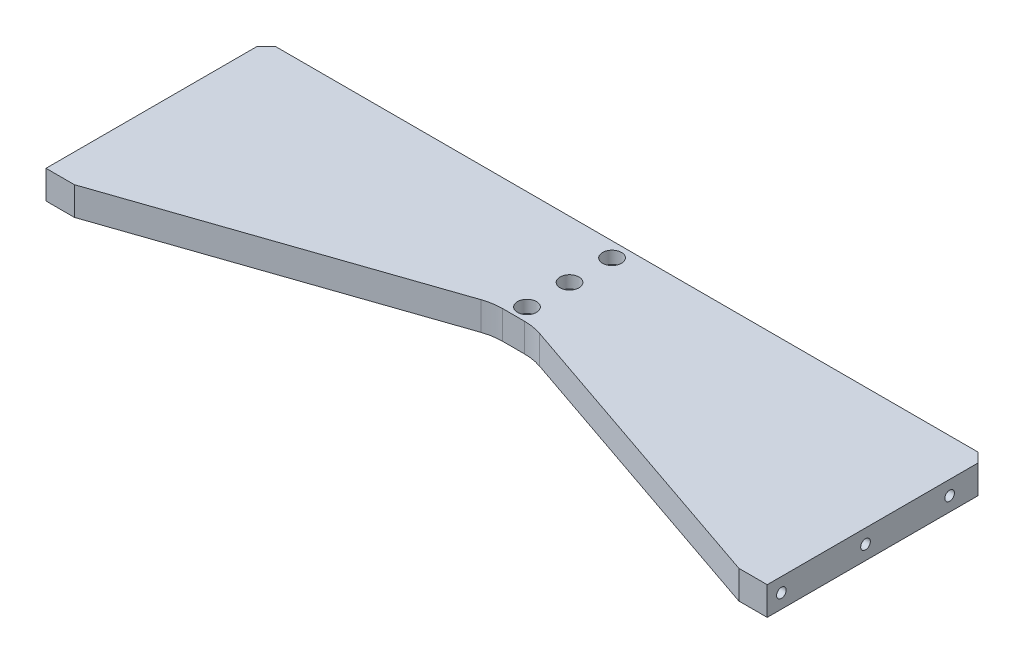
SolidWorks part; units mm, degrees
material "普通碳钢"
ref_plane "前视基准面" through (0, 0, 0) normal (0, 0, 1) x (1, 0, 0)
ref_plane "上视基准面" through (0, 0, 0) normal (0, 1, 0) x (1, 0, 0)
ref_plane "右视基准面" through (0, 0, 0) normal (1, 0, 0) x (0, 0, -1)
sketch "草图1" plane through (0, 0, 0) normal (0, 1, 0) x (1, 0, 0)
  line L1 (-381.5, -116.5) -> (381.5, -116.5)
  line L2 (-381.5, -116.5) -> (-381.5, 116.5)
  line L3 (-381.5, 116.5) -> (381.5, 116.5)
  line L4 (381.5, -116.5) -> (381.5, 116.5)
  line L5 (-381.5, -116.5) -> (381.5, 116.5) construction
  line L6 (-381.5, 116.5) -> (381.5, -116.5) construction
  point P0 (0, 0)
  dimension "D1" = 763
  dimension "D2" = 233
extrude "凸台-拉伸1" add sketch "草图1" along normal blind 30
chamfer "倒角1" distance 10 angle 45 2 edges at (381.5, 15, -116.5) (-381.5, 15, -116.5)
sketch "草图2" plane through (0, 30, 0) normal (0, 1, 0) x (1, 0, 0)
  line L0 (-351.5, -116.5) -> (-21.5, -3.5)
  line L1 (-381.5, -116.5) -> (381.5, -116.5) construction
  line L2 (-21.5, -3.5) -> (21.5, -3.5)
  line L3 (21.5, -3.5) -> (351.5, -116.5)
  line L4 (-381.5, 106.5) -> (-381.5, -116.5) construction
  line L5 (381.5, -116.5) -> (381.5, 106.5) construction
  dimension "D1" = 360
  dimension "D2" = 360
  dimension "D3" = 30
  dimension "D4" = 30
  dimension "D5" = 113
extrude "切除-拉伸1" cut sketch "草图2" against normal blind 30 and the other way through all flip side to cut
fillet "圆角1" radius 60 2 edges at (21.5, 15, 3.5) (-21.5, 15, 3.5)
hole_wizard "打孔尺寸(%根据)内六角圆柱头螺钉的类型1" positions "草图3" profile "草图4" counterbore size "M12" standard "GB" end condition through all
sketch "草图3" plane through (0, 30, 0) normal (0, 1, 0) x (1, 0, 0)
  line L0 (381.5, -116.5) -> (381.5, 106.5) construction
  line L1 (351.5, -116.5) -> (381.5, -116.5) construction
  point P0 (0, 100.8621)
  point P2 (0, 55.8621)
  point P4 (0, 10.8621)
  dimension "D1" = 381.5
  dimension "D2" = 127.3621
  dimension "D3" = 172.3621
  dimension "D4" = 217.3621
sketch "草图4" plane through (0, 30, -100.8621) normal (1, 0, 0) x (0, 0, 1)
  line L0 (0, 0) -> (0, 30)
  line L1 (0, 30) -> (6.75, 30)
  line L3 (6.75, 30) -> (6.75, 13)
  line L4 (6.75, 13) -> (10, 13)
  line L5 (10, 13) -> (10, 0)
  line L7 (10, 0) -> (0, 0)
  line L11 (0, -6.35) -> (0, 107.95) construction
  dimension "通孔孔直径" = 13.5
  dimension "通孔孔深度" = 30
  dimension "柱形沉头孔直径" = 20
  dimension "柱形沉头孔深度" = 13
hole_wizard "M12 螺纹孔1" positions "草图5" profile "草图6" tap size "M12" standard "GB"
sketch "草图5" plane through (0, 0, -116.5) normal (0, 0, -1) x (-1, 0, 0)
  line L0 (-381.5, 0) -> (-381.5, 30) construction
  line L1 (381.5, 30) -> (381.5, 0) construction
  line L2 (351.5, 15) -> (251.0714, 15) construction
  line L3 (251.0714, 15) -> (150.6429, 15) construction
  line L4 (150.6429, 15) -> (50.2143, 15) construction
  line L5 (50.2143, 15) -> (-50.2143, 15) construction
  line L6 (-50.2143, 15) -> (-150.6429, 15) construction
  line L7 (-150.6429, 15) -> (-251.0714, 15) construction
  line L8 (-251.0714, 15) -> (-351.5, 15) construction
  point P0 (351.5, 15)
  point P2 (251.0714, 15)
  point P4 (150.6429, 15)
  point P6 (50.2143, 15)
  point P8 (-50.2143, 15)
  point P10 (-150.6429, 15)
  point P12 (-251.0714, 15)
  point P14 (-351.5, 15)
  point P38 (-381.5, 15)
  dimension "D1" = 30
  dimension "D2" = 30
sketch "草图6" plane through (-351.5, 15, -116.5) normal (1, 0, 0) x (0, 1, 0)
  line L0 (0, 0) -> (0, 32.3144)
  line L1 (0, 32.3144) -> (5.1, 29.25)
  line L2 (5.1, 29.25) -> (5.1, 0)
  line L5 (5.1, 0) -> (0, 0)
  line L10 (0, 32.3144) -> (-5.1, 29.25) construction
  line L11 (0, -6.35) -> (0, 107.95) construction
  dimension "螺纹孔钻头直径" = 10.2
  dimension "螺纹孔钻头深度" = 29.25
  dimension "导头角度" = 118
cosmetic thread "孔螺蚊线1" parameters "D1"=24, "D2"=12
cosmetic thread "孔螺蚊线2" parameters "D1"=24, "D2"=12
cosmetic thread "孔螺蚊线3" parameters "D1"=24, "D2"=12
cosmetic thread "孔螺蚊线4" parameters "D1"=24, "D2"=12
cosmetic thread "孔螺蚊线5" parameters "D1"=24, "D2"=12
cosmetic thread "孔螺蚊线6" parameters "D1"=24, "D2"=12
cosmetic thread "孔螺蚊线7" parameters "D1"=24, "D2"=12
cosmetic thread "孔螺蚊线8" parameters "D1"=24, "D2"=12
hole_wizard "M12 螺纹孔2" positions "草图7" profile "草图8" tap size "M12" standard "GB"
sketch "草图7" plane through (381.5, 0, 0) normal (1, 0, 0) x (0, 0, -1)
  line L0 (-116.5, 30) -> (-116.5, 0) construction
  line L1 (116.5, 30) -> (116.5, 0) construction
  line L2 (-116.5, 0) -> (106.5, 0) construction
  line L3 (-101.5, 15) -> (-12.5, 15) construction
  line L4 (-12.5, 15) -> (76.5, 15) construction
  point P0 (76.5, 15)
  point P2 (-12.5, 15)
  point P4 (-101.5, 15)
  dimension "D1" = 15
  dimension "D2" = 40
  dimension "D3" = 15
sketch "草图8" plane through (381.5, 15, -76.5) normal (0, 1, 0) x (0, 0, -1)
  line L0 (0, 0) -> (0, 32.3144)
  line L1 (0, 32.3144) -> (5.1, 29.25)
  line L2 (5.1, 29.25) -> (5.1, 0)
  line L5 (5.1, 0) -> (0, 0)
  line L10 (0, 32.3144) -> (-5.1, 29.25) construction
  line L11 (0, -6.35) -> (0, 107.95) construction
  dimension "螺纹孔钻头直径" = 10.2
  dimension "螺纹孔钻头深度" = 29.25
  dimension "导头角度" = 118
cosmetic thread "孔螺蚊线9" parameters "D1"=24, "D2"=12
cosmetic thread "孔螺蚊线10" parameters "D1"=24, "D2"=12
cosmetic thread "孔螺蚊线11" parameters "D1"=24, "D2"=12
hole_wizard "M12 螺纹孔3" positions "草图9" profile "草图10" tap size "M12" standard "GB"
sketch "草图9" plane through (-381.5, 0, 0) normal (-1, 0, 0) x (0, 0, 1)
  line L0 (-106.5, 30) -> (-106.5, 0) construction
  line L1 (-106.5, 30) -> (116.5, 30) construction
  point P0 (-76.5, 15)
  point P2 (12.5, 15)
  point P4 (101.5, 15)
  dimension "D1" = 30
  dimension "D2" = 119
  dimension "D3" = 208
  dimension "D4" = 15
sketch "草图10" plane through (-381.5, 15, -76.5) normal (0, 1, 0) x (0, 0, 1)
  line L0 (0, 0) -> (0, 32.3144)
  line L1 (0, 32.3144) -> (5.1, 29.25)
  line L2 (5.1, 29.25) -> (5.1, 0)
  line L5 (5.1, 0) -> (0, 0)
  line L10 (0, 32.3144) -> (-5.1, 29.25) construction
  line L11 (0, -6.35) -> (0, 107.95) construction
  dimension "螺纹孔钻头直径" = 10.2
  dimension "螺纹孔钻头深度" = 29.25
  dimension "导头角度" = 118
cosmetic thread "孔螺蚊线12" parameters "D1"=24, "D2"=12
cosmetic thread "孔螺蚊线13" parameters "D1"=24, "D2"=12
cosmetic thread "孔螺蚊线14" parameters "D1"=24, "D2"=12
